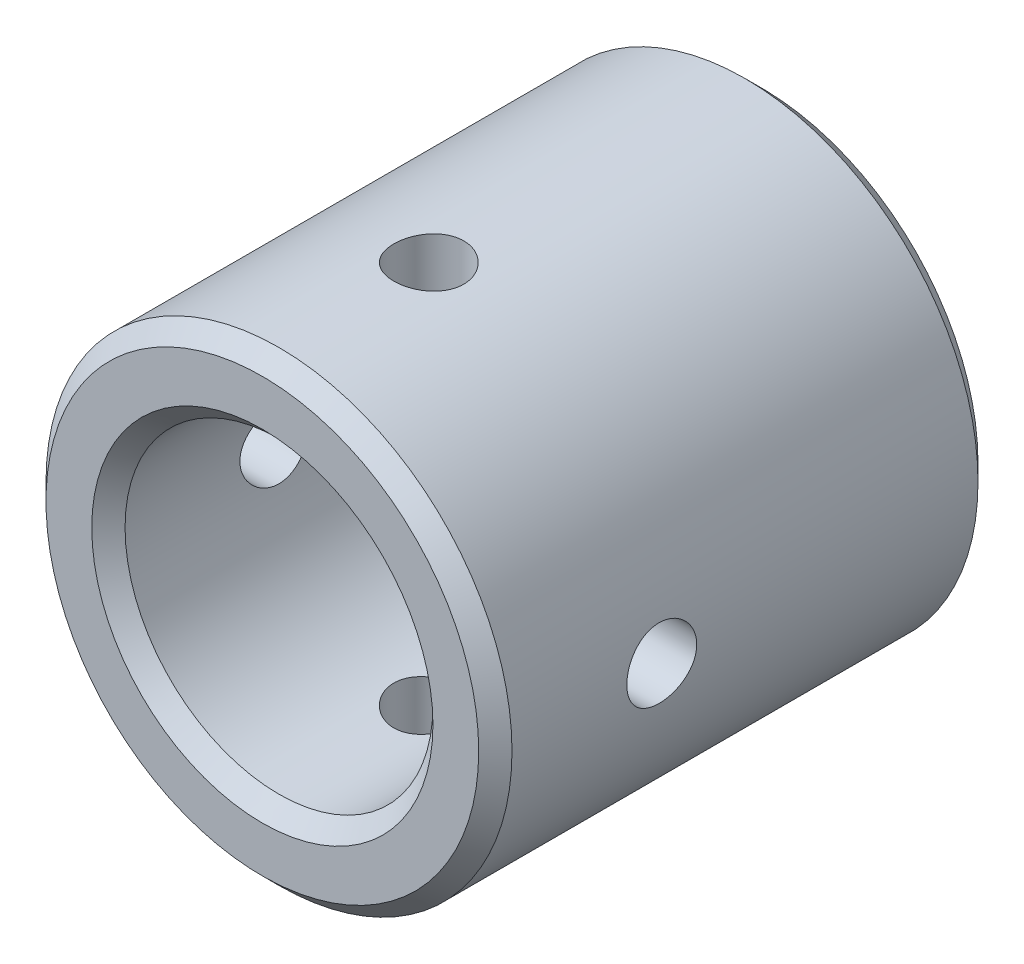
from build123d import *

# Parameters (mm, degrees)
SKETCH1_R             = 14
SKETCH1_R_2           = 9.25
BOSS_EXTRUDE1_DEPTH   = 15
SKETCH2_W             = 2.1
SKETCH2_H             = 14
SKETCH4_W             = 2.1
SKETCH4_H             = 14
M5_TAPPED_HOLE3_D     = 4.2
M5_TAPPED_HOLE4_D     = 4.2
M3_TAPPED_HOLE1_D     = 2.5
M3_TAPPED_HOLE1_DEPTH = 7.5
M3_TAPPED_HOLE1_TIP   = 0.751075774
CHAMFER1_SIZE         = 1


with BuildPart() as part:
    # Sketch1 → Boss-Extrude1 (new, symmetric)
    with BuildSketch(Plane.XY):
        Circle(SKETCH1_R)
        Circle(SKETCH1_R_2, mode=Mode.SUBTRACT)
    extrude(amount=BOSS_EXTRUDE1_DEPTH, both=True)

    # Sketch2 → M5 Tapped Hole1 (revolve, cut)
    with BuildSketch(Plane(origin=(0, 0, 5), x_dir=(0, 0, 1), z_dir=(1, 0, 0))):
        with Locations((1.05, 7)):
            Rectangle(SKETCH2_W, SKETCH2_H)
    revolve(axis=Axis((0, 6.35, 5), (0, -1, 0)), mode=Mode.SUBTRACT)

    # Sketch4 → M5 Tapped Hole2 (revolve, cut)
    with BuildSketch(Plane(origin=(0, 0, 5), x_dir=(0, 0, 1), z_dir=(0, 1, 0))):
        with Locations((1.05, 7)):
            Rectangle(SKETCH4_W, SKETCH4_H)
    revolve(axis=Axis((-6.35, 0, 5), (1, 0, 0)), mode=Mode.SUBTRACT)

    # M5 Tapped Hole3 (through all)
    with Locations(Plane.XZ):
        with Locations((0, 5)):
            Hole(M5_TAPPED_HOLE3_D / 2)

    # M5 Tapped Hole4 (through all)
    with Locations(Plane(origin=(0, 0, 0), x_dir=(0, 0, -1), z_dir=(1, 0, 0))):
        with Locations((-5, 0)):
            Hole(M5_TAPPED_HOLE4_D / 2)

    # M3 Tapped Hole1
    with Locations(Plane(origin=(0, 0, -15), x_dir=(-1, 0, 0), z_dir=(0, 0, -1))):
        with Locations((6, 10), (6, -10), (-6, -10), (-6, 10)):
            Hole(M3_TAPPED_HOLE1_D / 2, depth=M3_TAPPED_HOLE1_DEPTH)
            with Locations((0, 0, -(M3_TAPPED_HOLE1_DEPTH + M3_TAPPED_HOLE1_TIP / 2))):  # 118° drill point
                Cone(0, M3_TAPPED_HOLE1_D / 2, M3_TAPPED_HOLE1_TIP, mode=Mode.SUBTRACT)

    # Chamfer1
    chamfer1_edges = [part.edges().sort_by_distance(p)[0] for p in [
        (-14, 0, -15),
        (-14, 0, 15),
        (-9.25, 0, -15),
        (-9.25, 0, 15),
    ]]
    chamfer(chamfer1_edges, length=CHAMFER1_SIZE)


solid = part.part
